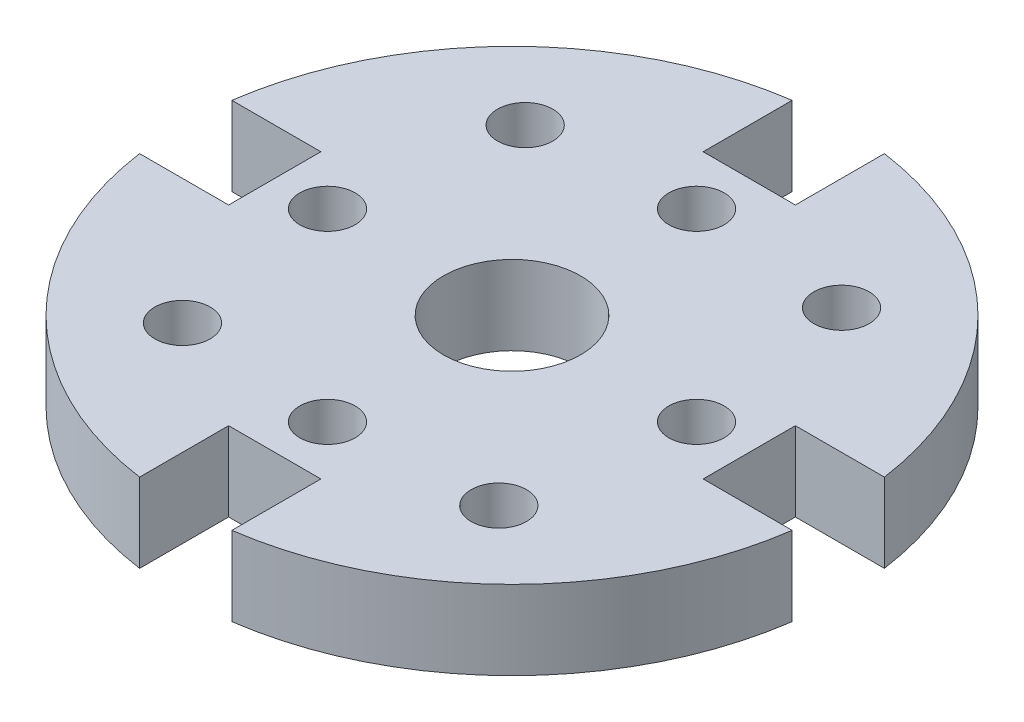
SolidWorks part; units mm, degrees
ref_plane "Front Plane" through (0, 0, 0) normal (0, 0, 1) x (1, 0, 0)
ref_plane "Top Plane" through (0, 0, 0) normal (0, 1, 0) x (1, 0, 0)
ref_plane "Right Plane" through (0, 0, 0) normal (1, 0, 0) x (0, 0, -1)
sketch "Sketch1" plane through (0, 0, 0) normal (0, 1, 0) x (1, 0, 0)
  line L0 (-45.4279, 0) -> (86.5356, 0) construction
  line L1 (0, 55.7505) -> (0, -37.9378) construction
  circle A0 centre (0, 0) radius 31.75
  circle A1 centre (-15.24, 16.51) radius 2.667
  circle A2 centre (15.24, 16.51) radius 2.667
  circle A3 centre (15.24, -16.51) radius 2.667
  circle A4 centre (-15.24, -16.51) radius 2.667
  dimension "D1" = 63.5
  dimension "D2" = 5.334
  dimension "D3" = 5.334
  dimension "D4" = 5.334
  dimension "D5" = 5.334
  dimension "D8" = 15.24
  dimension "D13" = 16.51
  dimension "D6" = 15.24
  dimension "D7" = 15.24
  dimension "D9" = 15.24
  dimension "D10" = 16.51
  dimension "D11" = 16.51
  dimension "D12" = 16.51
extrude "Boss-Extrude1" add sketch "Sketch1" against normal blind 7.62
sketch "Sketch2" plane through (0, 0, 0) normal (0, 1, 0) x (1, 0, 0)
  line L0 (-39.2664, 0) -> (68.4909, 0) construction
  line L1 (0, -47.5522) -> (0, 44.586) construction
  line L3 (-4.445, 40.64) -> (4.445, 40.64)
  line L4 (-4.445, 40.64) -> (-4.445, 22.86)
  line L5 (-4.445, 22.86) -> (4.445, 22.86)
  line L6 (4.445, 40.64) -> (4.445, 22.86)
  line L7 (-4.445, 40.64) -> (4.445, 22.86) construction
  line L8 (-4.445, 22.86) -> (4.445, 40.64) construction
  circle A0 centre (0, 0) radius 31.75 construction
  circle A1 centre (0, 0) radius 6.604
  point P6 (0, 31.75)
  point P30 (0, -5.715)
  dimension "D1" = 13.208
  dimension "D2" = 8.89
  dimension "D3" = 4.445
extrude "Cut-Extrude1" cut sketch "Sketch2" against normal through all
sketch "Sketch3" plane through (0, 0, 0) normal (0, 1, 0) x (1, 0, 0)
  circle A0 centre (-17.78, 0) radius 2.667
  circle A1 centre (0, 17.78) radius 2.667
  circle A2 centre (17.78, 0) radius 2.667
  circle A3 centre (0, -17.78) radius 2.667
  point P15 (0, 0)
  dimension "D1" = 5.334
  dimension "D3" = 17.78
  dimension "D4" = 4
extrude "Cut-Extrude2" cut sketch "Sketch3" against normal through all
pattern_circular "CirPattern1" count 4 every 90 about axis through (0, 0, 0) along (0, 1, 0) of "Cut-Extrude1"
scale "Scale1" bodies to scale 105 scale about origin uniform scaling yes scale factor 2
